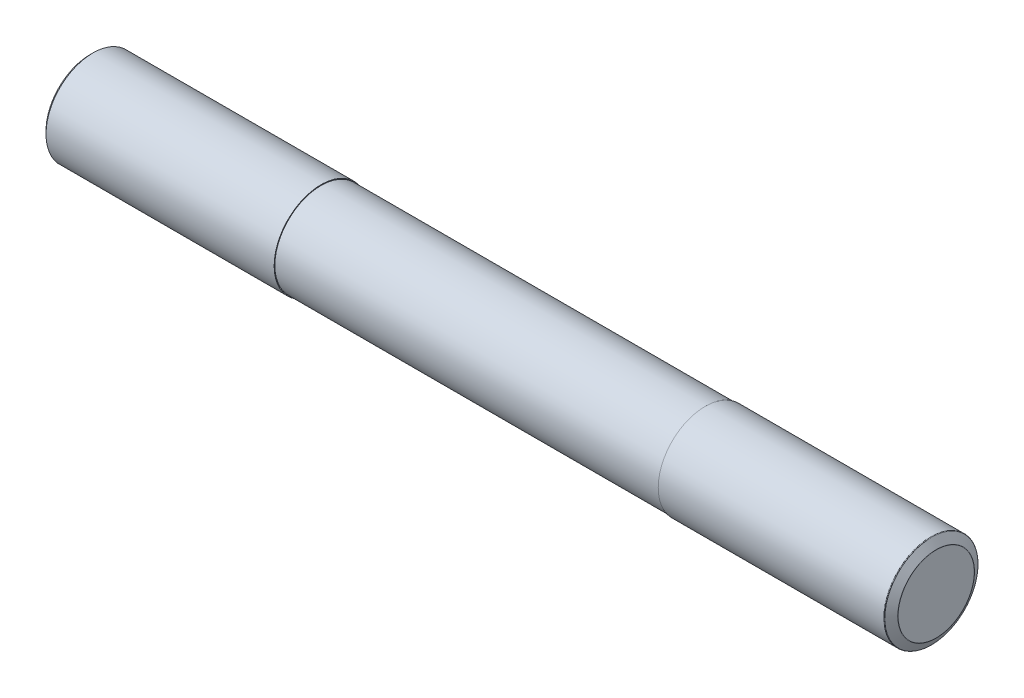
SolidWorks part; units mm, degrees
material "普通碳钢"
ref_plane "前视" through (0, 0, 0) normal (0, 0, 1) x (1, 0, 0)
ref_plane "上视" through (0, 0, 0) normal (0, 1, 0) x (1, 0, 0)
ref_plane "右视" through (0, 0, 0) normal (1, 0, 0) x (0, 0, -1)
sketch "草图1" plane through (0, 0, 0) normal (0, 0, 1) x (1, 0, 0)
  line L0 (-129.3158, 0) -> (129.0877, 0) construction
  line L1 (0, 80.6228) -> (0, -62.3772) construction
  line L2 (0, 32.5) -> (160, 32.5)
  line L3 (160, 32.5) -> (160, 32)
  line L4 (160, 32) -> (426, 32)
  line L5 (426, 32) -> (426, 32.5)
  line L6 (426, 32.5) -> (586, 32.5)
  line L7 (586, 32.5) -> (586, 0)
  line L8 (586, 0) -> (0, 0)
  line L9 (0, 0) -> (0, 32.5)
  dimension "D1" = 65
  dimension "D2" = 65
  dimension "D3" = 64
  dimension "D4" = 586
  dimension "D5" = 160
  dimension "D6" = 160
revolve "旋转1" add sketch "草图1" angle 360 about L0
chamfer "倒角1" distance 2 angle 45 1 edges at (0, 0, 32.5)
chamfer "倒角2" distance 6 angle 30 1 edges at (586, 0, 32.5)
fillet "圆角1" radius 0.5 2 edges at (582.5359, 0, 32.5) (586, 0, 26.5)
ref_plane "基准面1" through (0, -32.5, 0) normal (0, 1, 0) x (1, 0, 0)
hole_wizard "大小mm 暗销孔2" positions "草图7" profile "草图5" hole size "Ø12.0" standard "GB"
sketch "草图7" plane through (0, -32.5, 0) normal (0, 1, 0) x (1, 0, 0)
  line L0 (-50, 0) -> (50, 0) construction
  line L1 (0, 30.5) -> (0, -30.5) construction
  point P0 (77, 0)
  dimension "D1" = 77
sketch "草图5" plane through (77, -32.5, 0) normal (1, 0, 0) x (0, 0, -1)
  line L0 (0, 0) -> (0, 13.6052)
  line L1 (0, 13.6052) -> (6, 10)
  line L2 (6, 10) -> (6, 1.7321)
  line L3 (6, 1.7321) -> (9, 0)
  line L5 (9, 0) -> (0, 0)
  line L6 (-6, 1.7321) -> (-9, 0) construction
  line L10 (0, 13.6052) -> (-6, 10) construction
  line L11 (0, -6.35) -> (0, 107.95) construction
  dimension "孔直径" = 12
  dimension "孔深度" = 10
  dimension "近端锥形沉头孔直径" = 18
  dimension "近端锥形沉头孔角度" = 120
  dimension "导头角度" = 118
